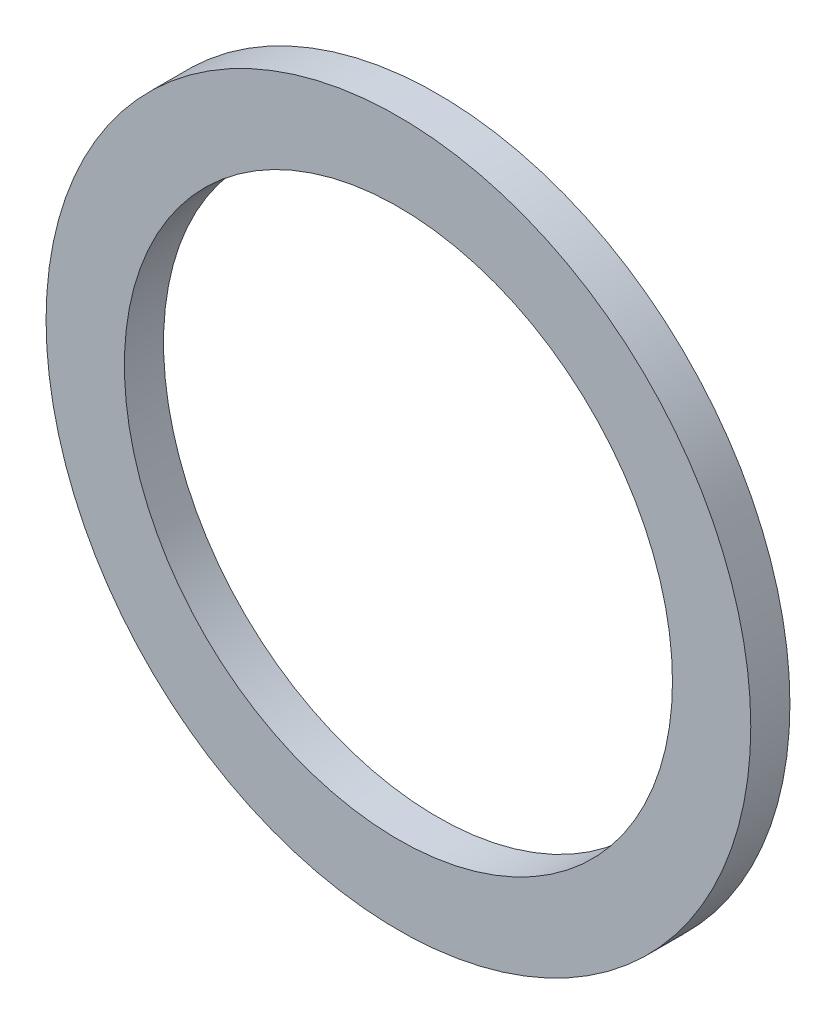
from build123d import *

# Parameters (mm, degrees)
SKETCH_1_R      = 22.5
SKETCH_1_R_2    = 17.5
EXTRUDE_1_DEPTH = 2.5


with BuildPart() as part:
    # 草图1 → 凸台-拉伸1 (new body)
    with BuildSketch(Plane.XY):
        Circle(SKETCH_1_R)
        Circle(SKETCH_1_R_2, mode=Mode.SUBTRACT)
    extrude(amount=EXTRUDE_1_DEPTH)


solid = part.part
